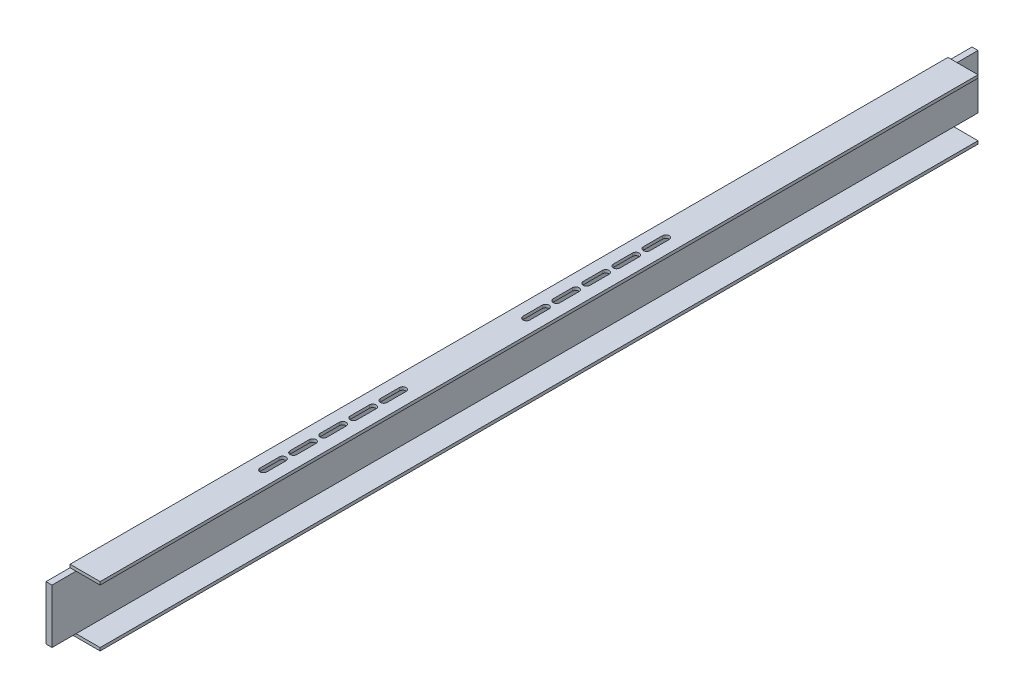
from build123d import *

# Parameters (mm, degrees)
EXTRUDE1_DEPTH         = 1232
SKETCH2_W              = 32
SKETCH2_H              = 32
CUT_EXTRUDE1_DEPTH     = 1236.242486316
SKETCH3_W              = 32
SKETCH3_H              = 4
CUT_EXTRUDE2_DEPTH     = 1200
CUT_EXTRUDE3_DEPTH     = 10
LPATTERN1_COUNT        = 5
LPATTERN1_PITCH        = 40
LPATTERN2_COUNT        = 2
LPATTERN2_PITCH        = 350
LPATTERN2_COPY_1_DEPTH = 10
LPATTERN2_COPY_2_DEPTH = 10
LPATTERN2_COPY_3_DEPTH = 10
LPATTERN2_COPY_4_DEPTH = 10


with BuildPart() as part:
    # Sketch1 → Extrude1 (new body)
    with BuildSketch(Plane.XY):
        Polygon((0, 0), (-40, 0), (-40, 80), (0, 80), (0, 76), (-32, 76), (-32, 4), (0, 4), align=None)
    extrude(amount=EXTRUDE1_DEPTH)

    # Sketch2 → Cut-Extrude1 (cut, through all)
    with BuildSketch(Plane(origin=(0, 80, 0), x_dir=(1, 0, 0), z_dir=(0, 1, 0))):
        with Locations((-16, -16)):
            Rectangle(SKETCH2_W, SKETCH2_H)
        with Locations((-16, -1216)):
            Rectangle(SKETCH2_W, SKETCH2_H)
    extrude(amount=-CUT_EXTRUDE1_DEPTH, mode=Mode.SUBTRACT)

    # Sketch3 → Cut-Extrude2 (cut)
    with BuildSketch(Plane(origin=(-32, 0, 0), x_dir=(0, 0, -1), z_dir=(1, 0, 0))):
        with Locations((-1216, 78)):
            Rectangle(SKETCH3_W, SKETCH3_H)
        with Locations((-1216, 2)):
            Rectangle(SKETCH3_W, SKETCH3_H)
        with Locations((-16, 78)):
            Rectangle(SKETCH3_W, SKETCH3_H)
        with Locations((-16, 2)):
            Rectangle(SKETCH3_W, SKETCH3_H)
    extrude(amount=-CUT_EXTRUDE2_DEPTH, mode=Mode.SUBTRACT)

    # Sketch4 → Cut-Extrude3 (cut)
    with BuildSketch(Plane(origin=(0, 80, 0), x_dir=(1, 0, 0), z_dir=(0, 1, 0))):
        with BuildLine():
            Line((-24.5, -937.25), (-24.5, -962.75))
            ThreePointArc((-24.5, -962.75), (-20, -967.25), (-15.5, -962.75))
            Line((-15.5, -962.75), (-15.5, -937.25))
            ThreePointArc((-15.5, -937.25), (-20, -932.75), (-24.5, -937.25))
        make_face()
    cut_extrude3 = extrude(amount=-CUT_EXTRUDE3_DEPTH, mode=Mode.SUBTRACT)

    # LPattern1: Cut-Extrude3 ×5
    with Locations(*[(0, 0, -i * LPATTERN1_PITCH) for i in range(1, LPATTERN1_COUNT)]):
        add(cut_extrude3, mode=Mode.SUBTRACT)

    # LPattern2: Cut-Extrude3 ×2
    with Locations(*[(0, 0, -i * LPATTERN2_PITCH) for i in range(1, LPATTERN2_COUNT)]):
        add(cut_extrude3, mode=Mode.SUBTRACT)

    # LPattern2 copy 1 sketch → LPattern2 copy 1 (cut)
    with BuildSketch(Plane(origin=(0, 80, -390), x_dir=(1, 0, 0), z_dir=(0, 1, 0))):
        with BuildLine():
            Line((-24.5, -937.25), (-24.5, -962.75))
            ThreePointArc((-24.5, -962.75), (-20, -967.25), (-15.5, -962.75))
            Line((-15.5, -962.75), (-15.5, -937.25))
            ThreePointArc((-15.5, -937.25), (-20, -932.75), (-24.5, -937.25))
        make_face()
    extrude(amount=-LPATTERN2_COPY_1_DEPTH, mode=Mode.SUBTRACT)

    # LPattern2 copy 2 sketch → LPattern2 copy 2 (cut)
    with BuildSketch(Plane(origin=(0, 80, -430), x_dir=(1, 0, 0), z_dir=(0, 1, 0))):
        with BuildLine():
            Line((-24.5, -937.25), (-24.5, -962.75))
            ThreePointArc((-24.5, -962.75), (-20, -967.25), (-15.5, -962.75))
            Line((-15.5, -962.75), (-15.5, -937.25))
            ThreePointArc((-15.5, -937.25), (-20, -932.75), (-24.5, -937.25))
        make_face()
    extrude(amount=-LPATTERN2_COPY_2_DEPTH, mode=Mode.SUBTRACT)

    # LPattern2 copy 3 sketch → LPattern2 copy 3 (cut)
    with BuildSketch(Plane(origin=(0, 80, -470), x_dir=(1, 0, 0), z_dir=(0, 1, 0))):
        with BuildLine():
            Line((-24.5, -937.25), (-24.5, -962.75))
            ThreePointArc((-24.5, -962.75), (-20, -967.25), (-15.5, -962.75))
            Line((-15.5, -962.75), (-15.5, -937.25))
            ThreePointArc((-15.5, -937.25), (-20, -932.75), (-24.5, -937.25))
        make_face()
    extrude(amount=-LPATTERN2_COPY_3_DEPTH, mode=Mode.SUBTRACT)

    # LPattern2 copy 4 sketch → LPattern2 copy 4 (cut)
    with BuildSketch(Plane(origin=(0, 80, -510), x_dir=(1, 0, 0), z_dir=(0, 1, 0))):
        with BuildLine():
            Line((-24.5, -937.25), (-24.5, -962.75))
            ThreePointArc((-24.5, -962.75), (-20, -967.25), (-15.5, -962.75))
            Line((-15.5, -962.75), (-15.5, -937.25))
            ThreePointArc((-15.5, -937.25), (-20, -932.75), (-24.5, -937.25))
        make_face()
    extrude(amount=-LPATTERN2_COPY_4_DEPTH, mode=Mode.SUBTRACT)


solid = part.part
